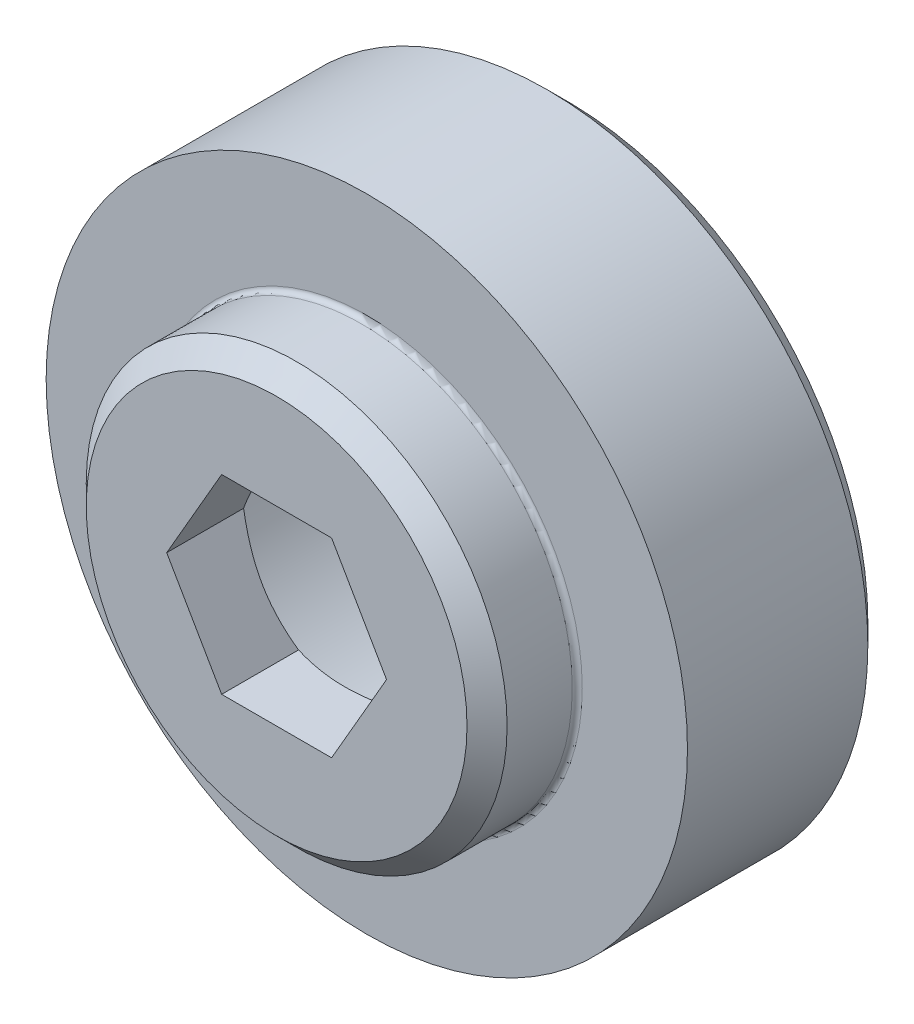
from build123d import *

# Parameters (mm, degrees)
SKETCH_1_R              = 32
EXTRUDE_1_DEPTH         = 20
SKETCH_2_R              = 21
EXTRUDE_2_DEPTH         = 9
HOLE_WIZARD_M48_1_D     = 43
HOLE_WIZARD_M48_1_DEPTH = 15
HOLE_WIZARD_M48_1_TIP   = 12.918503309
CUT_EXTRUDE_1_DEPTH     = 54.749418602
CHAMFER_2_SIZE          = 2
CHAMFER_3_SIZE          = 2
FILLET_1_R              = 0.5


with BuildPart() as part:
    # 草图1 → 凸台-拉伸1 (new body)
    with BuildSketch(Plane.XY):
        Circle(SKETCH_1_R)
    extrude(amount=EXTRUDE_1_DEPTH)

    # 草图2 → 凸台-拉伸2 (add)
    with BuildSketch(Plane.XY.offset(20)):
        Circle(SKETCH_2_R)
    extrude(amount=EXTRUDE_2_DEPTH)

    # M48 螺纹孔1
    with Locations(Plane(origin=(0, 0, 0), x_dir=(-1, 0, 0), z_dir=(0, 0, -1))):
        with Locations((0, 0)):
            Hole(HOLE_WIZARD_M48_1_D / 2, depth=HOLE_WIZARD_M48_1_DEPTH)
            with Locations((0, 0, -(HOLE_WIZARD_M48_1_DEPTH + HOLE_WIZARD_M48_1_TIP / 2))):  # 118° drill point
                Cone(0, HOLE_WIZARD_M48_1_D / 2, HOLE_WIZARD_M48_1_TIP, mode=Mode.SUBTRACT)

    # 草图5 → 切除-拉伸1 (cut, through all)
    with BuildSketch(Plane.XY.offset(29)):
        Polygon((10.969655115, 0), (5.484827557, 9.5), (-5.484827557, 9.5), (-10.969655115, 0), (-5.484827557, -9.5), (5.484827557, -9.5), align=None)
    extrude(amount=-CUT_EXTRUDE_1_DEPTH, mode=Mode.SUBTRACT)

    # 倒角2
    chamfer_2_edges = [part.edges().sort_by_distance(p)[0] for p in [
        (-32, 0, 0),
    ]]
    chamfer(chamfer_2_edges, length=CHAMFER_2_SIZE)

    # 倒角3
    chamfer_3_edges = [part.edges().sort_by_distance(p)[0] for p in [
        (-21, 0, 29),
    ]]
    chamfer(chamfer_3_edges, length=CHAMFER_3_SIZE)

    # 圆角1
    fillet_1_edges = [part.edges().sort_by_distance(p)[0] for p in [
        (-21, 0, 20),
    ]]
    fillet(fillet_1_edges, radius=FILLET_1_R)


solid = part.part
